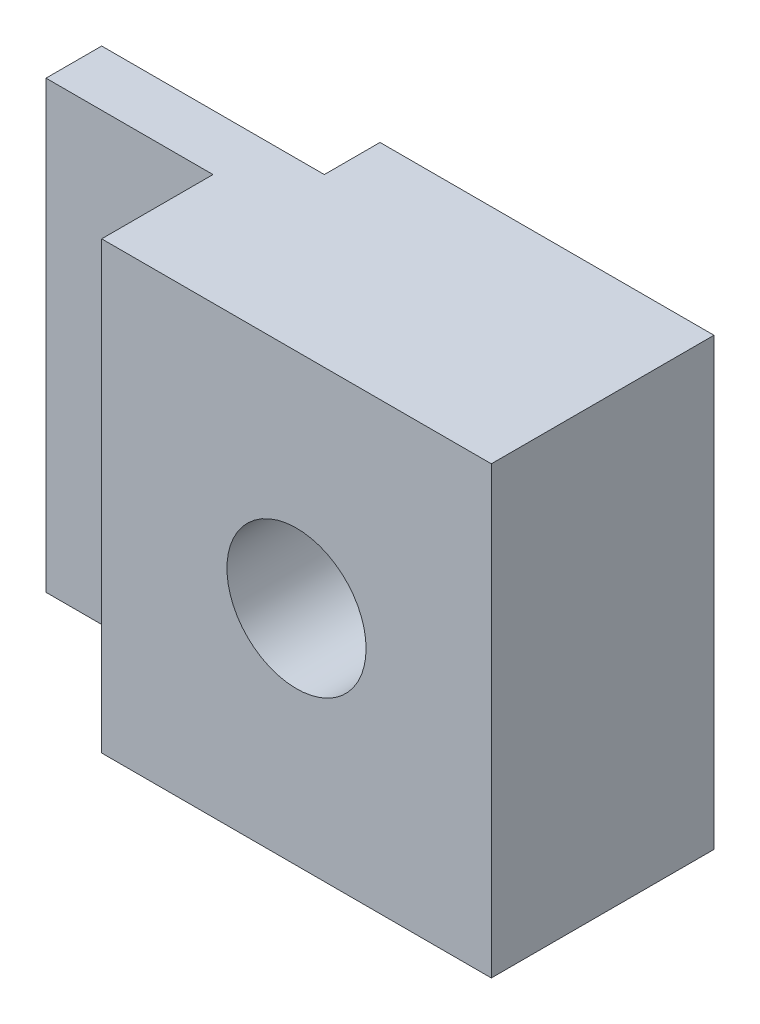
SolidWorks part; units mm, degrees
ref_plane "Front Plane" through (0, 0, 0) normal (0, 0, 1) x (1, 0, 0)
ref_plane "Top Plane" through (0, 0, 0) normal (0, 1, 0) x (1, 0, 0)
ref_plane "Right Plane" through (0, 0, 0) normal (1, 0, 0) x (0, 0, -1)
sketch "Sketch1" plane through (0, 0, 0) normal (0, 0, 1) x (1, 0, 0)
  line L1 (0, 0) -> (12, 0)
  line L2 (0, 0) -> (0, -8)
  line L3 (0, -8) -> (12, -8)
  line L4 (12, 0) -> (12, -8)
extrude "Boss-Extrude1" add sketch "Sketch1" along normal blind 2
sketch "Sketch2" plane through (0, 0, 2) normal (0, 0, 1) x (1, 0, 0)
  line L0 (12, 0) -> (0, 0) construction
  line L1 (12, -8) -> (5, -8)
  line L2 (12, -8) -> (12, 0)
  line L3 (12, 0) -> (5, 0)
  line L4 (5, -8) -> (5, 0)
extrude "Boss-Extrude2" add sketch "Sketch2" along normal blind 2
sketch "Sketch3" plane through (0, 0, 4) normal (0, 0, 1) x (1, 0, 0)
  line L0 (8.5, 0) -> (8.5, -8) construction
  line L1 (12, 0) -> (5, 0) construction
  line L2 (5, -8) -> (12, -8) construction
  circle A0 centre (8.5, -4) radius 1.25
  dimension "D1" = 2.5
extrude "Cut-Extrude1" cut sketch "Sketch3" against normal blind 10
sketch "Sketch4" plane through (0, 0, 0) normal (0, 0, -1) x (-1, 0, 0)
  line L0 (0, 0) -> (0, -8) construction
  line L2 (0, -4) -> (0, 1.1737)
  line L3 (0, 1.1737) -> (-6, 1.1737)
  line L4 (-6, -4) -> (-6, 1.1737)
  line L7 (-6, -4) -> (-6, -6.5)
  line L8 (-6, -6.5) -> (0, -6.5)
  line L9 (0, -4) -> (0, -6.5)
extrude "Cut-Extrude2" cut sketch "Sketch4" against normal blind 1
sketch "Sketch5" plane through (0, 0, 0) normal (0, 0, -1) x (-1, 0, 0)
  line L0 (0, 0) -> (-6, 0) construction
  line L1 (0, -8) -> (-2, -8)
  line L2 (0, -8) -> (0, 0)
  line L3 (0, 0) -> (-2, 0)
  line L4 (-2, -8) -> (-2, 0)
extrude "Cut-Extrude3" cut sketch "Sketch5" against normal blind 7
other "Move Face1" face at (9.75, -4, 4) parameters "D1"=0.5
hole_wizard "M3 Tapped Hole4" positions "Sketch6" profile "Sketch7" tap size "M3" standard "GB"
sketch "Sketch6" plane through (0, 0, 4) normal (0, 0, 1) x (1, 0, 0)
  point P0 (8.5, -4)
sketch "Sketch7" plane through (8.5, -4, 4) normal (1, 0, 0) x (0, -1, 0)
  line L0 (0, 0) -> (0, 8.2511)
  line L1 (0, 8.2511) -> (1.25, 7.5)
  line L2 (1.25, 7.5) -> (1.25, 0)
  line L5 (1.25, 0) -> (0, 0)
  line L10 (0, 8.2511) -> (-1.25, 7.5) construction
  line L11 (0, -6.35) -> (0, 107.95) construction
  dimension "螺纹孔钻头直径" = 2.5
  dimension "螺纹孔钻头深度" = 7.5
  dimension "导头角度" = 118
cosmetic thread "Cosmetic thread 2" parameters "D1"=4, "D2"=3
